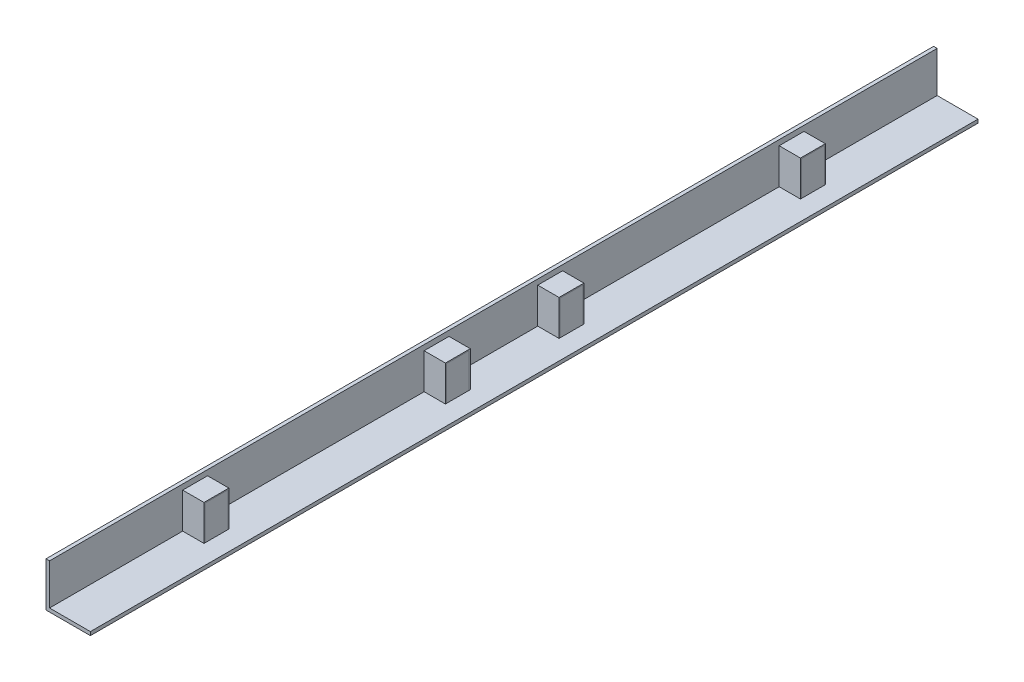
from build123d import *

# Parameters (mm, degrees)
EXTRUDE_1_DEPTH        = 1250
EXTRUDE_1_2_DEPTH      = 60
SKETCH_3_W             = 64
SKETCH_3_H             = 97
EXTRUDE_2_DEPTH        = 3
PATTERN_LINEAR_1_COUNT = 2
PATTERN_LINEAR_1_PITCH = 680
SKETCH_4_W             = 46
SKETCH_4_H             = 60
CUT_EXTRUDE_1_DEPTH    = 10


with BuildPart() as part:
    # 草图1 → Extrude 1 (new, symmetric)
    with BuildSketch(Plane.XY):
        Polygon((0, 125), (10, 125), (10, 10), (125, 10), (125, 0), (0, 0), align=None)
    extrude(amount=EXTRUDE_1_DEPTH, both=True)

    # 草图4 → 切除-拉伸1 (cut)
    with BuildSketch(Plane.XZ):
        with Locations((44, 160)):
            Rectangle(SKETCH_4_W, SKETCH_4_H)
        with Locations((44, 840)):
            Rectangle(SKETCH_4_W, SKETCH_4_H)
        with Locations((44, -840)):
            Rectangle(SKETCH_4_W, SKETCH_4_H)
        with Locations((44, -160)):
            Rectangle(SKETCH_4_W, SKETCH_4_H)
    extrude(amount=-CUT_EXTRUDE_1_DEPTH, mode=Mode.SUBTRACT)


with BuildPart() as body_2:
    # 草图2 → Extrude 1 2 (new body)
    with BuildSketch(Plane(origin=(10, 0, 0), x_dir=(0, 0, -1), z_dir=(1, 0, 0))):
        Polygon((-872, 10), (-872, 107), (-808, 107), (-808, 10), (-805, 10), (-805, 110), (-875, 110), (-875, 10), align=None)
    extrude(amount=EXTRUDE_1_2_DEPTH)


with BuildPart() as body_3:
    # 草图3 → 凸台-拉伸2 (new body)
    with BuildSketch(Plane(origin=(70, 0, 0), x_dir=(0, 0, -1), z_dir=(1, 0, 0))):
        with Locations((-840, 58.5)):
            Rectangle(SKETCH_3_W, SKETCH_3_H)
    extrude(amount=-EXTRUDE_2_DEPTH)


with BuildPart() as pattern_linear_1_1:
    # 阵列(线性)1: pattern copy
    add(body_2.part.moved(Location(Vector(0, 0, -1) * (1 * PATTERN_LINEAR_1_PITCH))))


with BuildPart() as pattern_linear_1_2:
    # 阵列(线性)1: pattern copy
    add(body_3.part.moved(Location(Vector(0, 0, -1) * (1 * PATTERN_LINEAR_1_PITCH))))


with BuildPart() as body_6:
    # 镜向1: mirrored copy
    add(pattern_linear_1_2.part.mirror(Plane.XY))


with BuildPart() as body_7:
    # Mirror 1 2: mirrored copy
    add(body_2.part.mirror(Plane.XY))


with BuildPart() as body_8:
    # Mirror 1 3: mirrored copy
    add(pattern_linear_1_1.part.mirror(Plane.XY))


with BuildPart() as body_9:
    # Mirror 1 4: mirrored copy
    add(body_3.part.mirror(Plane.XY))


solid = Compound([part.part, body_2.part, body_3.part, pattern_linear_1_1.part, pattern_linear_1_2.part, body_6.part, body_7.part, body_8.part, body_9.part])
